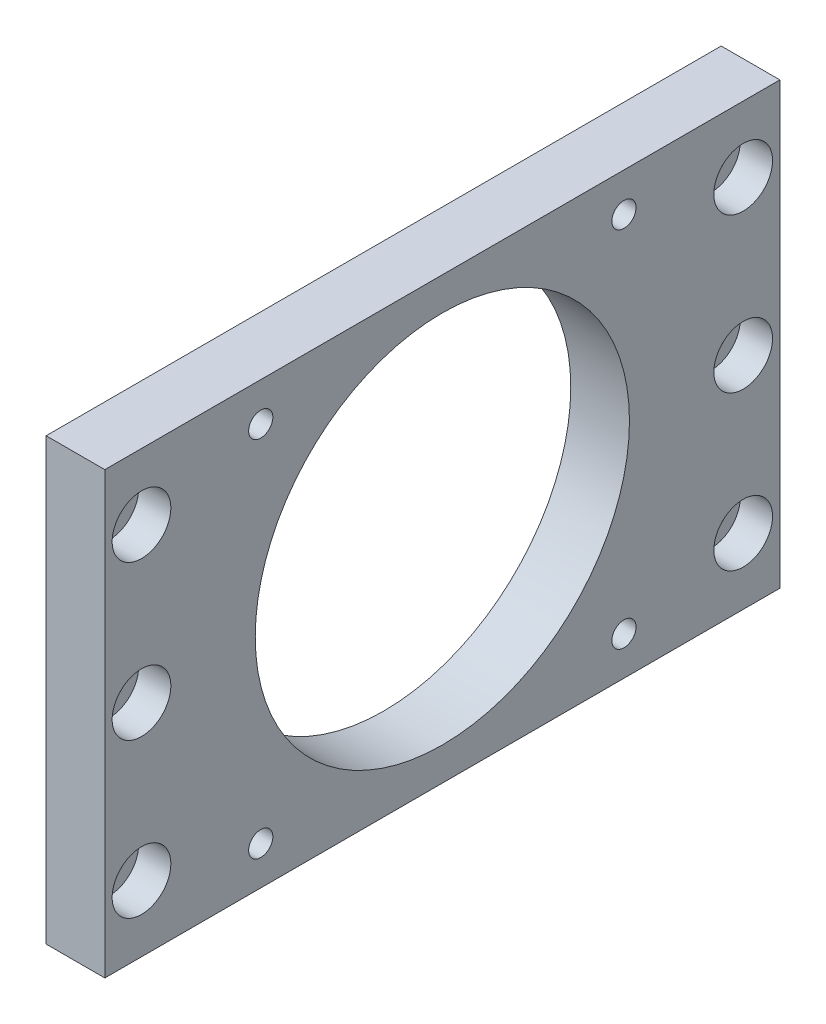
SolidWorks part; units mm, degrees
ref_plane "Front Plane" through (0, 0, 0) normal (0, 0, 1) x (1, 0, 0)
ref_plane "Top Plane" through (0, 0, 0) normal (0, 1, 0) x (1, 0, 0)
ref_plane "Right Plane" through (0, 0, 0) normal (1, 0, 0) x (0, 0, -1)
sketch "Sketch1" plane through (0, 0, 0) normal (1, 0, 0) x (0, 0, -1)
  line L1 (-46, 30) -> (46, 30)
  line L2 (-46, 30) -> (-46, -30)
  line L3 (-46, -30) -> (46, -30)
  line L4 (46, 30) -> (46, -30)
  line L5 (-46, 30) -> (46, -30) construction
  line L6 (-46, -30) -> (46, 30) construction
  point P0 (0, 0)
  dimension "D1" = 92
  dimension "D2" = 60
extrude "Boss-Extrude1" add sketch "Sketch1" along normal mid plane 8
hole_wizard "M4 Tapped Hole1" positions "Sketch2" profile "Sketch3" tap size "M4" standard "ISO"
sketch "Sketch2" plane through (4, 0, 0) normal (1, 0, 0) x (0, 0, -1)
  line L0 (0, 0) -> (0, 39.1456) construction
  line L2 (0, 0) -> (56.8125, 0) construction
  point P0 (-24.75, 24.75)
  point P2 (24.75, 24.75)
  point P4 (-24.75, -24.75)
  point P6 (24.75, -24.75)
  dimension "D1" = 49.5
  dimension "D2" = 49.5
sketch "Sketch3" plane through (4, 24.75, 24.75) normal (0, 1, 0) x (0, 0, -1)
  line L0 (0, 0) -> (0, 11.0914)
  line L1 (0, 11.0914) -> (1.65, 10.1)
  line L2 (1.65, 10.1) -> (1.65, 0)
  line L5 (1.65, 0) -> (0, 0)
  line L10 (0, 11.0914) -> (-1.65, 10.1) construction
  line L11 (0, -6.35) -> (0, 107.95) construction
  dimension "螺纹孔钻头直径" = 3.3
  dimension "螺纹孔钻头深度" = 10.1
  dimension "导头角度" = 118
cosmetic thread "Cosmetic Thread1" parameters "D1"=8, "D2"=4
cosmetic thread "Cosmetic Thread2" parameters "D1"=8, "D2"=4
cosmetic thread "Cosmetic Thread3" parameters "D1"=8, "D2"=4
cosmetic thread "Cosmetic Thread4" parameters "D1"=8, "D2"=4
sketch "Sketch4" plane through (4, 0, 0) normal (1, 0, 0) x (0, 0, -1)
  circle A0 centre (0, 0) radius 25.5
  dimension "D1" = 51
extrude "Cut-Extrude1" cut sketch "Sketch4" against normal through all
hole_wizard "CBORE for M4 Hex Socket Head Cap Screw1" positions "Sketch5" profile "Sketch6" counterbore size "M4" standard "ISO" end condition through all
sketch "Sketch5" plane through (4, 0, 0) normal (1, 0, 0) x (0, 0, -1)
  line L0 (0, 0) -> (0, 34.3902) construction
  line L2 (0, 0) -> (17.9593, 0) construction
  point P0 (-41, 21)
  point P2 (-41, 0)
  point P4 (-41, -21)
  point P6 (41, 21)
  point P8 (41, 0)
  point P10 (41, -21)
  dimension "D1" = 42
  dimension "D2" = 82
sketch "Sketch6" plane through (4, 21, 41) normal (0, 1, 0) x (0, 0, -1)
  line L0 (0, 0) -> (0, 8)
  line L1 (0, 8) -> (2.25, 8)
  line L3 (2.25, 8) -> (2.25, 4.4)
  line L4 (2.25, 4.4) -> (4, 4.4)
  line L5 (4, 4.4) -> (4, 0)
  line L7 (4, 0) -> (0, 0)
  line L11 (0, -6.35) -> (0, 107.95) construction
  dimension "通孔孔直径" = 4.5
  dimension "通孔孔深度" = 8
  dimension "柱形沉头孔直径" = 8
  dimension "柱形沉头孔深度" = 4.4
hole_wizard "M4 Tapped Hole2" positions "Sketch7" profile "Sketch8" tap size "M4" standard "ISO"
sketch "Sketch7" plane through (0, -30, 0) normal (0, -1, 0) x (-1, 0, 0)
  point P0 (0, -34)
  point P3 (0, 34)
sketch "Sketch8" plane through (0, -30, 34) normal (1, 0, 0) x (0, 0, -1)
  line L0 (0, 0) -> (0, 11.0914)
  line L1 (0, 11.0914) -> (1.65, 10.1)
  line L2 (1.65, 10.1) -> (1.65, 0)
  line L5 (1.65, 0) -> (0, 0)
  line L10 (0, 11.0914) -> (-1.65, 10.1) construction
  line L11 (0, -6.35) -> (0, 107.95) construction
  dimension "螺纹孔钻头直径" = 3.3
  dimension "螺纹孔钻头深度" = 10.1
  dimension "导头角度" = 118
cosmetic thread "Cosmetic Thread7" parameters "D1"=8, "D2"=4.3
cosmetic thread "Cosmetic Thread8" parameters "D1"=8, "D2"=4.3
